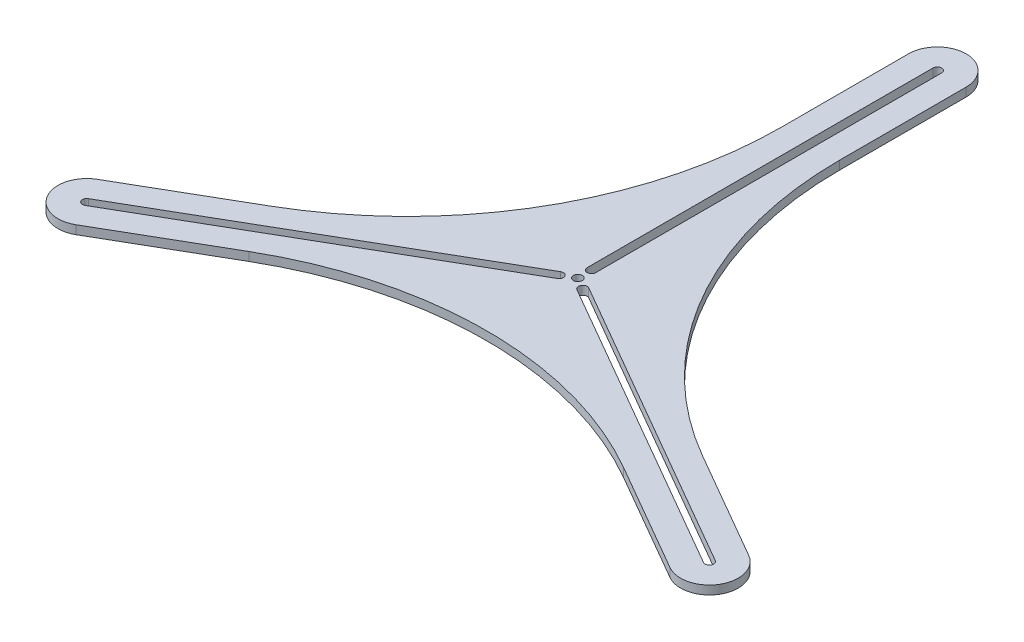
from build123d import *

# Parameters (mm, degrees)
SKETCH1_R           = 3.1
BOSS_EXTRUDE2_DEPTH = 6


with BuildPart() as part:
    # Sketch1 → Boss-Extrude2 (new body)
    with BuildSketch(Plane(origin=(0, 0, 0), x_dir=(1, 0, 0), z_dir=(0, 1, 0))):
        with BuildLine():
            Line((-7.442631645, 168.908075373), (-7.442631645, 256.750012922))
            ThreePointArc((-7.442631645, 256.750012922), (12.557368355, 276.750012922), (32.557368355, 256.750012922))
            Line((32.557368355, 256.750012922), (32.557368355, 168.908075373))
            ThreePointArc((32.557368355, 168.908075373), (67.390763371, 38.908075373), (162.557368355, -56.258529611))
            Line((162.557368355, -56.258529611), (238.63071779, -100.179498385))
            ThreePointArc((238.63071779, -100.179498385), (245.951225865, -127.500006461), (218.63071779, -134.820514537))
            Line((218.63071779, -134.820514537), (142.557368355, -90.899545762))
            ThreePointArc((142.557368355, -90.899545762), (12.557368355, -56.066150746), (-117.442631645, -90.899545762))
            Line((-117.442631645, -90.899545762), (-193.51598108, -134.820514537))
            ThreePointArc((-193.51598108, -134.820514537), (-220.836485566, -127.499986835), (-213.515954749, -100.179483183))
            Line((-213.515954749, -100.179483183), (-137.442631645, -56.258529611))
            ThreePointArc((-137.442631645, -56.258529611), (-42.276026661, 38.908075373), (-7.442631645, 168.908075373))
        make_face()
        with Locations(Location((12.557368355, 7.25, 0), (0, 0, 270))):
            Circle(SKETCH1_R, mode=Mode.SUBTRACT)
        with BuildLine():
            Line((5.830127019, -0.098076211), (-202.015969889, -120.098076211))
            ThreePointArc((-202.015969889, -120.098076211), (-206.114046101, -119), (-205.015969889, -114.901923789))
            Line((-205.015969889, -114.901923789), (2.830127019, 5.098076211))
            ThreePointArc((2.830127019, 5.098076211), (6.92820323, 4), (5.830127019, -0.098076211))
        make_face(mode=Mode.SUBTRACT)
        with BuildLine():
            Line((22.284609691, 5.098076211), (230.130706599, -114.901923789))
            ThreePointArc((230.130706599, -114.901923789), (231.22878281, -119), (227.130706599, -120.098076211))
            Line((227.130706599, -120.098076211), (19.284609691, -0.098076211))
            ThreePointArc((19.284609691, -0.098076211), (18.186533479, 4), (22.284609691, 5.098076211))
        make_face(mode=Mode.SUBTRACT)
        with BuildLine():
            Line((9.557368355, 16.75), (9.557368355, 256.75))
            ThreePointArc((9.557368355, 256.75), (12.557368355, 259.75), (15.557368355, 256.75))
            Line((15.557368355, 256.75), (15.557368355, 16.75))
            ThreePointArc((15.557368355, 16.75), (12.557368355, 13.75), (9.557368355, 16.75))
        make_face(mode=Mode.SUBTRACT)
    extrude(amount=BOSS_EXTRUDE2_DEPTH)


solid = part.part
